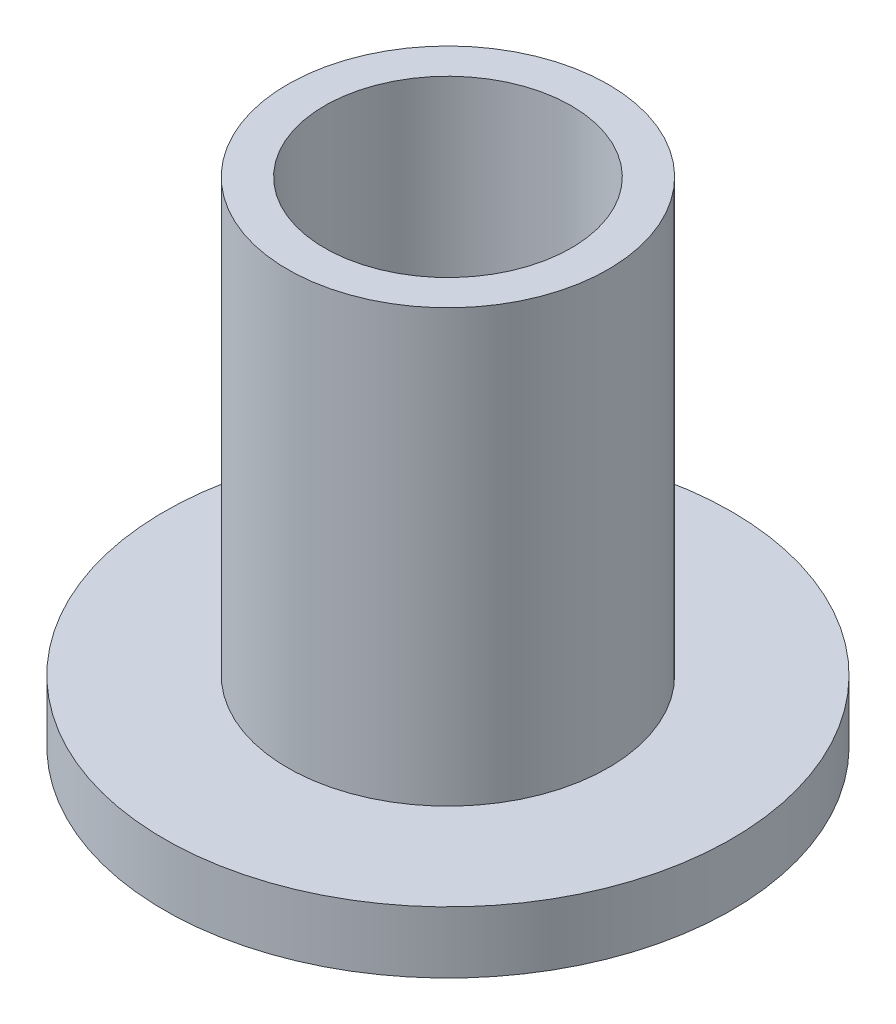
SolidWorks part; units mm, degrees
ref_plane "前视基准面" through (0, 0, 0) normal (0, 0, 1) x (1, 0, 0)
ref_plane "上视基准面" through (0, 0, 0) normal (0, 1, 0) x (1, 0, 0)
ref_plane "右视基准面" through (0, 0, 0) normal (1, 0, 0) x (0, 0, -1)
sketch "草图1" plane through (0, 0, 0) normal (0, 0, 1) x (1, 0, 0)
  line L0 (-10, 0) -> (-23, 0)
  line L1 (-23, 0) -> (-23, 5)
  line L2 (-23, 5) -> (-13, 5)
  line L3 (-13, 5) -> (-13, 40)
  line L4 (-13, 40) -> (-10, 40)
  line L5 (-10, 40) -> (-10, 0)
  line L6 (0, 0) -> (0, 55.7641) construction
  dimension "D1" = 10
  dimension "D2" = 5
  dimension "D3" = 3
  dimension "D4" = 35
  dimension "D5" = 10
revolve "旋转1" add sketch "草图1" angle 360 about L6
